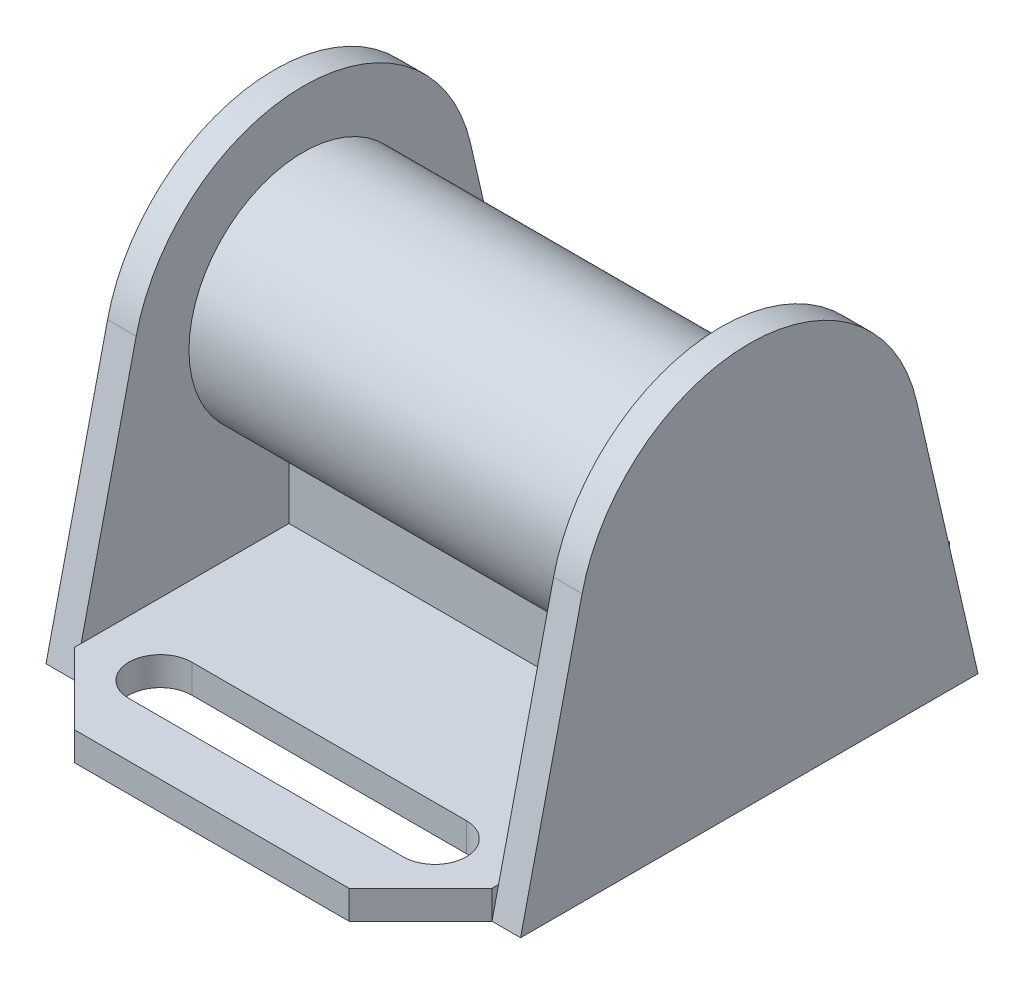
from build123d import *

# Parameters (mm, degrees)
EXTRUDE_1_DEPTH      = 10
EXTRUDE_2_DEPTH      = 10
EXTRUDE_3_DEPTH      = 73
EXTRUDE_3_DEPTH_BACK = 73
SKETCH_3_R           = 40
SKETCH_3_R_2         = 32
EXTRUDE_4_REACH      = 188.585
EXTRUDE_4_END_RADIUS = 40
SKETCH_4_W           = 146
SKETCH_4_H           = 10


with BuildPart() as part:
    # 草图1 → 凸台-拉伸1 (new body)
    with BuildSketch(Plane(origin=(0, 0, 0), x_dir=(1, 0, 0), z_dir=(0, 1, 0))):
        Polygon((-73, -80), (-73, 80), (-48, 105), (48, 105), (73, 80), (73, -80), (48, -105), (-48, -105), align=None)
        with BuildLine():
            Line((-48, 86), (48, 86))
            ThreePointArc((48, 86), (59, 75), (48, 64))
            Line((48, 64), (-48, 64))
            ThreePointArc((-48, 64), (-59, 75), (-48, 86))
        make_face(mode=Mode.SUBTRACT)
        with BuildLine():
            Line((-48, -86), (48, -86))
            ThreePointArc((48, -86), (59, -75), (48, -64))
            Line((48, -64), (-48, -64))
            ThreePointArc((-48, -64), (-59, -75), (-48, -86))
        make_face(mode=Mode.SUBTRACT)
    extrude(amount=EXTRUDE_1_DEPTH)


with BuildPart() as body_2:
    # 草图2 → 凸台-拉伸2 (new body)
    with BuildSketch(Plane.ZY.offset(73)):
        with BuildLine():
            Line((-80, 0), (-58.468736425, 93.468736425))
            ThreePointArc((-58.468736425, 93.468736425), (0, 140), (58.468736425, 93.468736425))
            Line((58.468736425, 93.468736425), (80, 0))
            Line((80, 0), (-80, 0))
        make_face()
    extrude(amount=EXTRUDE_2_DEPTH)


with BuildPart() as body_3:
    # 镜向1: mirrored copy
    add(body_2.part.mirror(Plane(origin=(0, 0, 0), x_dir=(0, 0, 1), z_dir=(1, 0, 0))))


with BuildPart() as body_4:
    # 草图3 → 凸台-拉伸3 (new, two sides: drawn at the far end of the back side and taken through both)
    with BuildSketch(Plane(origin=(0, 0, 0), x_dir=(0, 0, -1), z_dir=(1, 0, 0)).offset(-EXTRUDE_3_DEPTH_BACK)):
        with Locations((0, 80)):
            Circle(SKETCH_3_R)
        with Locations((0, 80)):
            Circle(SKETCH_3_R_2, mode=Mode.SUBTRACT)
    extrude(amount=EXTRUDE_3_DEPTH + EXTRUDE_3_DEPTH_BACK)


with BuildPart() as body_5:
    # 凸台-拉伸4: up to this cylinder (the profile starts outside it)
    extrude_4_end = Plane(origin=(0, 80, 0), z_dir=(1, 0, 0)) * Cylinder(EXTRUDE_4_END_RADIUS, 458.17, mode=Mode.PRIVATE)
    # 草图4 → 凸台-拉伸4 (new, up to the surface)
    with BuildSketch(Plane(origin=(0, 10, 0), x_dir=(1, 0, 0), z_dir=(0, 1, 0)), mode=Mode.PRIVATE) as extrude_4_sk1:
        Rectangle(SKETCH_4_W, SKETCH_4_H)
    extrude_4_tool1 = extrude(extrude_4_sk1.sketch, amount=EXTRUDE_4_REACH, mode=Mode.PRIVATE) - extrude_4_end
    add(extrude_4_tool1.solids().sort_by_distance((0, 10, 0))[0])


solid = Compound([part.part, body_2.part, body_3.part, body_4.part, body_5.part])
